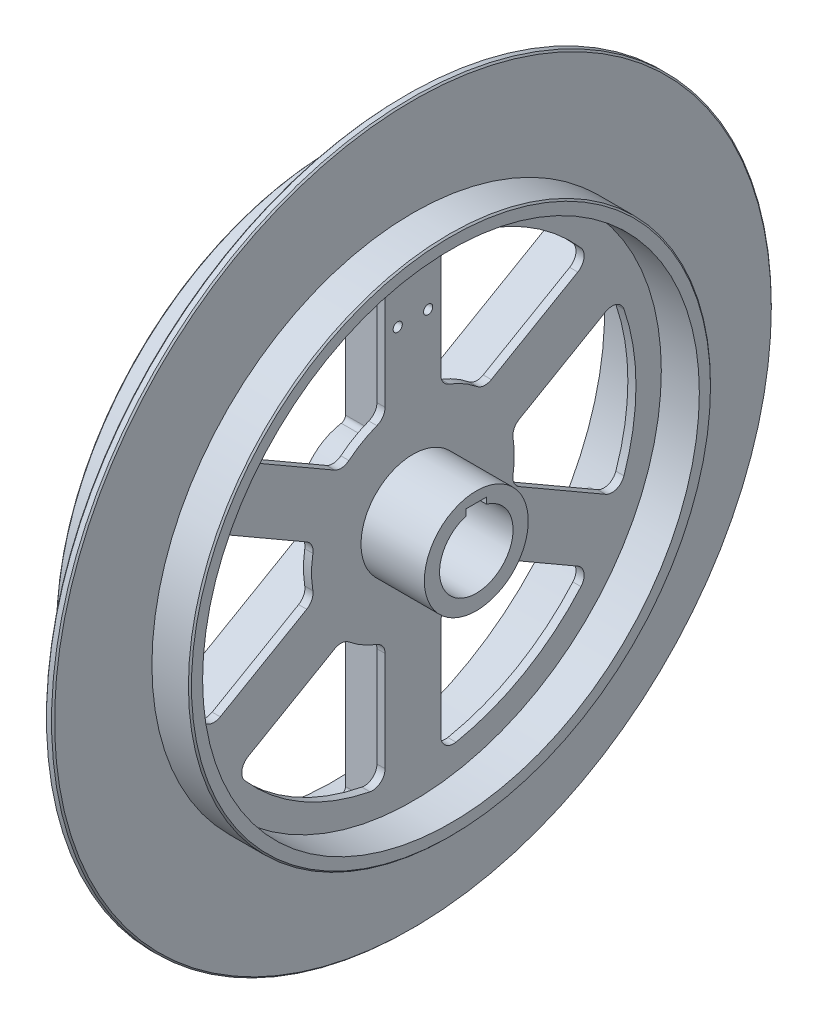
SolidWorks part; units mm, degrees
material "45"
ref_plane "Front Plane" through (0, 0, 0) normal (0, 0, 1) x (1, 0, 0)
ref_plane "Top Plane" through (0, 0, 0) normal (0, 1, 0) x (1, 0, 0)
ref_plane "Right Plane" through (0, 0, 0) normal (1, 0, 0) x (0, 0, -1)
sketch "Sketch1" plane through (0, 0, 0) normal (0, 0, 1) x (1, 0, 0)
  line L0 (-31, 550) -> (-31, 534)
  line L1 (109, 710) -> (125, 710)
  line L4 (79, 137.5) -> (79, 102.5)
  line L5 (125, 710) -> (125, 515)
  line L7 (109, 710) -> (109, 550)
  line L8 (-373.3517, 0) -> (373.3517, 0) construction
  line L9 (125, 490) -> (125, 102.5)
  line L10 (109, 534) -> (109, 137.5)
  line L11 (125, 102.5) -> (250, 102.5)
  line L12 (79, 137.5) -> (109, 137.5)
  line L13 (-31, 550) -> (109, 550)
  line L14 (-31, 534) -> (109, 534)
  line L15 (125, 515) -> (200, 515)
  line L16 (125, 490) -> (200, 490)
  line L17 (0, 102.5) -> (79, 102.5)
  line L18 (0, 72.5) -> (250, 72.5)
  line L19 (125, 102.5) -> (250, 102.5)
  line L20 (200, 515) -> (200, 490)
  line L21 (250, 102.5) -> (250, 72.5)
  line L22 (0, 102.5) -> (0, 72.5)
  dimension "D1" = 125
  dimension "D2" = 16
  dimension "D3" = 1030
  dimension "D4" = 25
  dimension "D5" = 1420
  dimension "D6" = 1100
  dimension "D7" = 140
  dimension "D8" = 275
  dimension "D9" = 30
  dimension "D10" = 250
  dimension "D11" = 145
  dimension "D12" = 30
  dimension "D13" = 75
  dimension "D14" = 16
revolve "Revolve1" add sketch "Sketch1" angle 360 about L8
sketch "Sketch3" plane through (109, 0, 0) normal (-1, 0, 0) x (0, 0, 1)
  line L0 (-55, 407.2162) -> (-55, 210.2974)
  line L1 (-154.6229, 152.7801) -> (-325.1595, 251.2395)
  line L2 (0, 0) -> (0, 655.2261) construction
  arc A0 (-71.1111, 186.931) -> (-126.3315, 155.0495) centre (0, 0) ccw
  arc A1 (-331.4945, 289.3293) -> (-84.8193, 431.7473) centre (0, 0) cw
  circle A2 centre (0, 0) radius 534 construction
  arc A3 (-55, 210.2974) -> (-71.1111, 186.931) centre (-80, 210.2974) cw
  arc A4 (-126.3315, 155.0495) -> (-154.6229, 152.7801) centre (-142.1229, 174.4307) cw
  arc A5 (-55, 407.2162) -> (-84.8193, 431.7473) centre (-80, 407.2162) ccw
  arc A6 (-325.1595, 251.2395) -> (-331.4945, 289.3293) centre (-312.6595, 272.8901) cw
  dimension "D1" = 200
  dimension "D2" = 440
  dimension "D5" = 25
  dimension "D3" = 110
  dimension "D4" = 60
extrude "Cut-Extrude1" cut sketch "Sketch3" against normal through all
pattern_circular "CirPattern1" count 6 over 360 about axis through (0, 0, 0) along (1, 0, 0) of "Cut-Extrude1"
sketch "Sketch4" plane through (109, 0, 0) normal (-1, 0, 0) x (0, 0, 1)
  line L0 (-8, 533.9401) -> (-8, 102.1873)
  line L1 (8, 533.9401) -> (8, 102.1873)
  line L2 (0, 0) -> (0, 614.7598) construction
  circle A1 centre (0, 0) radius 102.5 construction
  circle A3 centre (0, 0) radius 102.5 construction
  circle A4 centre (0, 0) radius 534 construction
  circle A5 centre (0, 0) radius 534 construction
  arc A6 (8, 533.9401) -> (-8, 533.9401) centre (0, 0) ccw
  arc A7 (8, 102.1873) -> (-8, 102.1873) centre (0, 0) ccw
  dimension "D1" = 16
extrude "Boss-Extrude1" add sketch "Sketch4" along normal up to surface (109 mm away) up to face at (0, 0, 72.5)
fillet "Fillet2" radius 10 8 edges at (109, 335.6036, -8) (94, 137.2671, -8) (39.5, 102.1873, -8) (39.5, 102.1873, 8) (94, 137.2671, 8) (109, 335.6036, 8) (54.5, 533.9401, 8) (54.5, 533.9401, -8)
pattern_circular "CirPattern2" count 6 over 360 about axis through (0, 0, 0) along (1, 0, 0) of "Boss-Extrude1", "Fillet2"
sketch "Sketch5" plane through (109, 0, 0) normal (-1, 0, 0) x (0, 0, 1)
  line L1 (-30, 425) -> (30, 425) construction
  line L2 (-30, 425) -> (-30, 335) construction
  line L3 (-30, 335) -> (30, 335) construction
  line L4 (30, 425) -> (30, 335) construction
  line L5 (-30, 425) -> (30, 335) construction
  line L6 (-30, 335) -> (30, 425) construction
  circle A0 centre (-30, 425) radius 9
  circle A1 centre (-30, 335) radius 9
  circle A2 centre (30, 335) radius 9
  circle A3 centre (30, 425) radius 9
  point P0 (0, 380)
  dimension "D3" = 18
  dimension "D1" = 60
  dimension "D2" = 90
  dimension "D4" = 380
extrude "Cut-Extrude2" cut sketch "Sketch5" against normal through all
sketch "Sketch6" plane through (0, 0, 8) normal (0, 0, 1) x (1, 0, 0)
  line L0 (109, 533.6907) -> (109, 136.3167) construction
  line L1 (94, 380) -> (40.8749, 380) construction
  line L2 (94, 395) -> (109, 395)
  line L3 (109, 395) -> (109, 365)
  line L4 (109, 365) -> (94, 365)
  arc A0 (94, 395) -> (94, 365) centre (94, 380) ccw
  dimension "D1" = 30
extrude "Cut-Extrude3" cut sketch "Sketch6" against normal through all and the other way blind 20
chamfer "Chamfer1" distance 3 angle 45 4 edges at (200, 0, 515) (125, 0, 710) (-31, 0, 550) (109, 0, 710)
sketch "Sketch7" plane through (0, 0, 0) normal (-1, 0, 0) x (0, 0, 1)
  line L1 (-20, 81.9) -> (20, 81.9)
  line L2 (-20, 81.9) -> (-20, 63.1)
  line L3 (-20, 63.1) -> (20, 63.1)
  line L4 (20, 81.9) -> (20, 63.1)
  line L5 (-20, 81.9) -> (20, 63.1) construction
  line L6 (-20, 63.1) -> (20, 81.9) construction
  circle A0 centre (0, 0) radius 72.5 construction
  point P0 (0, 72.5)
  dimension "D1" = 40
  dimension "D2" = 9.4
extrude "Cut-Extrude4" cut sketch "Sketch7" against normal through all
